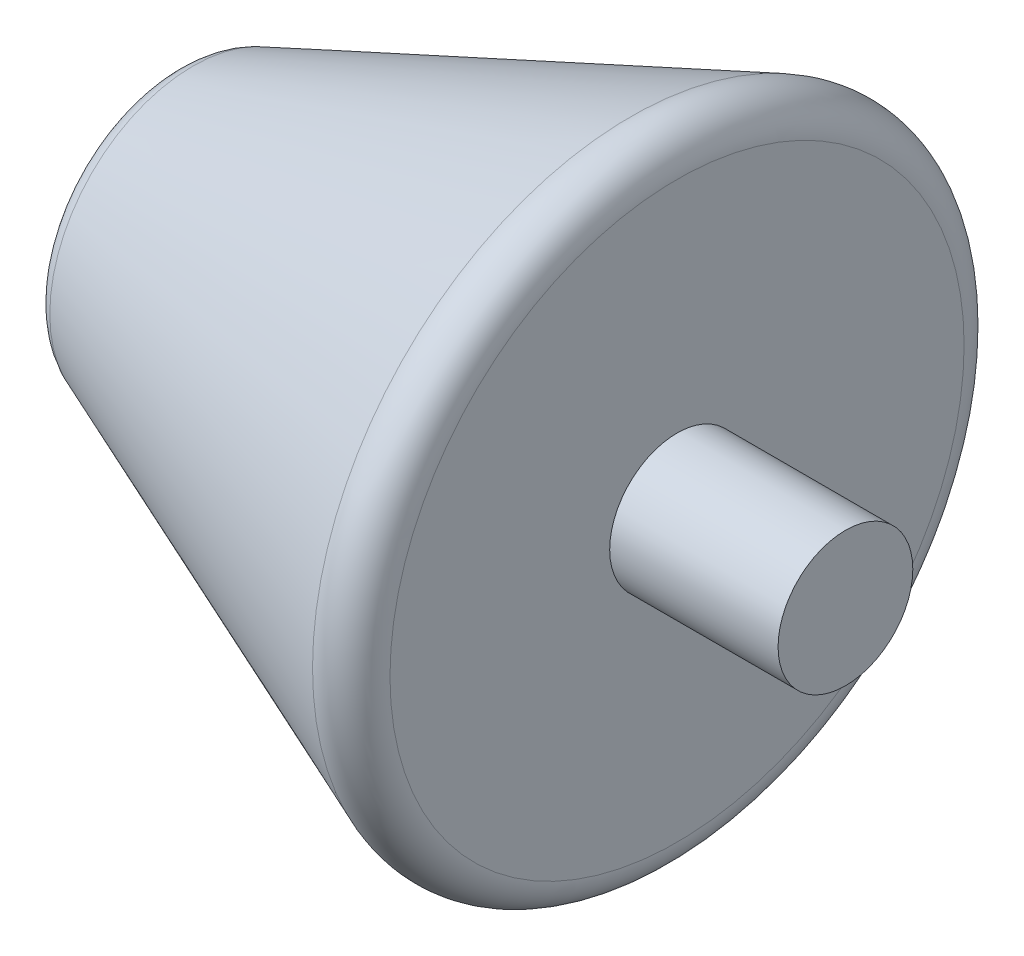
from build123d import *

# Parameters (mm, degrees)
FILLET1_R           = 2
SKETCH2_R           = 4
BOSS_EXTRUDE1_DEPTH = 10
FILLET2_R           = 2


with BuildPart() as part:
    # Sketch1 → Revolve1 (revolve)
    with BuildSketch(Plane.XY, mode=Mode.PRIVATE) as revolve1_sk:
        Polygon((30, 20), (30, 0), (0, 0), (0, 8), align=None)
    revolve(revolve1_sk.sketch.rotate(Axis((10.657678515, 0, 0), (1, 0, 0)), 90), axis=Axis((10.657678515, 0, 0), (1, 0, 0)))

    # Fillet1
    fillet1_edges = [part.edges().sort_by_distance(p)[0] for p in [
        (0, 0, -8),
    ]]
    fillet(fillet1_edges, radius=FILLET1_R)

    # Sketch2 → Boss-Extrude1 (add)
    with BuildSketch(Plane(origin=(30, 0, 0), x_dir=(0, 0, -1), z_dir=(1, 0, 0))):
        with Locations(Location((0, 0, 0), (0, 0, 180))):
            Circle(SKETCH2_R)
    extrude(amount=BOSS_EXTRUDE1_DEPTH)

    # Fillet2
    fillet2_edges = [part.edges().sort_by_distance(p)[0] for p in [
        (30, 0, -20),
    ]]
    fillet(fillet2_edges, radius=FILLET2_R)


solid = part.part
